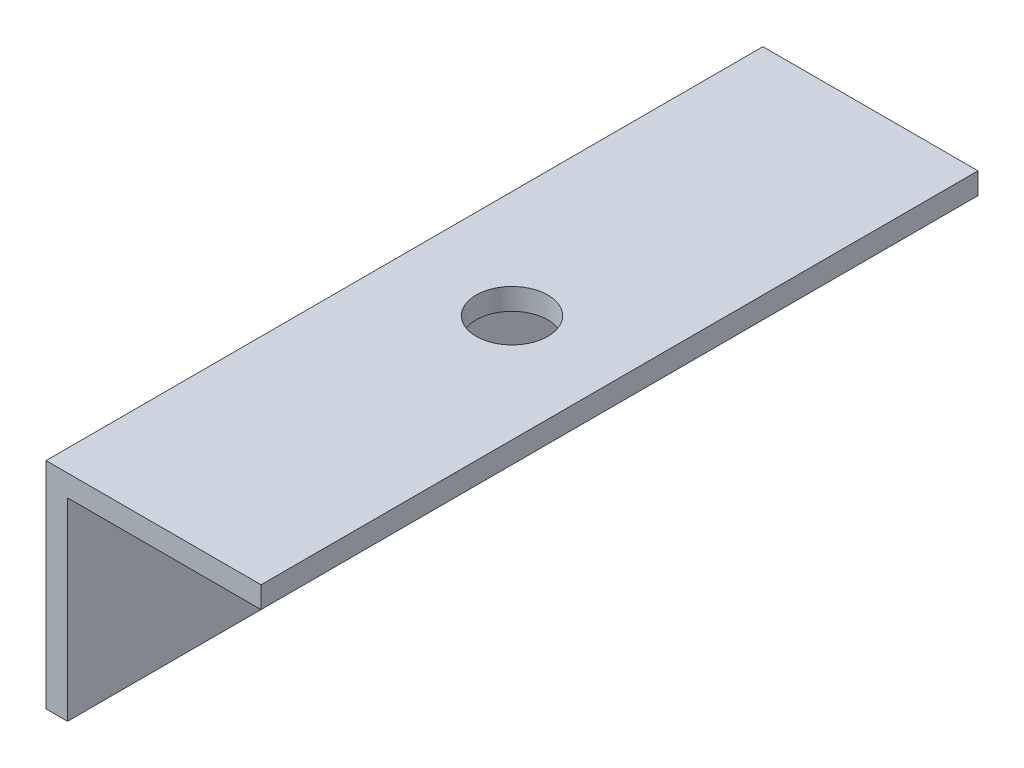
SolidWorks part; units mm, degrees
ref_plane "前视基准面" through (0, 0, 0) normal (0, 0, 1) x (1, 0, 0)
ref_plane "上视基准面" through (0, 0, 0) normal (0, 1, 0) x (1, 0, 0)
ref_plane "右视基准面" through (0, 0, 0) normal (1, 0, 0) x (0, 0, -1)
sketch "草图1" plane through (0, 0, 0) normal (0, 0, 1) x (1, 0, 0)
  line L0 (0, 0) -> (30, 0)
  line L1 (0, 0) -> (0, -30)
  line L2 (3, -3) -> (3, -30)
  line L3 (3, -3) -> (30, -3)
  line L4 (30, -3) -> (30, 0)
  line L5 (0, -30) -> (3, -30)
  dimension "D1" = 3
extrude "凸台-拉伸1" add sketch "草图1" along normal blind 100
sketch "草图2" plane through (0, 0, 0) normal (0, 1, 0) x (1, 0, 0)
  line L0 (15, 0) -> (15, -100)
  line L1 (30, 0) -> (0, 0) construction
  line L2 (30, -100) -> (0, -100) construction
  circle A0 centre (15, -50) radius 5
extrude "切除-拉伸1" cut sketch "草图2" against normal blind 10 contours L0 A0 | L0 A0
